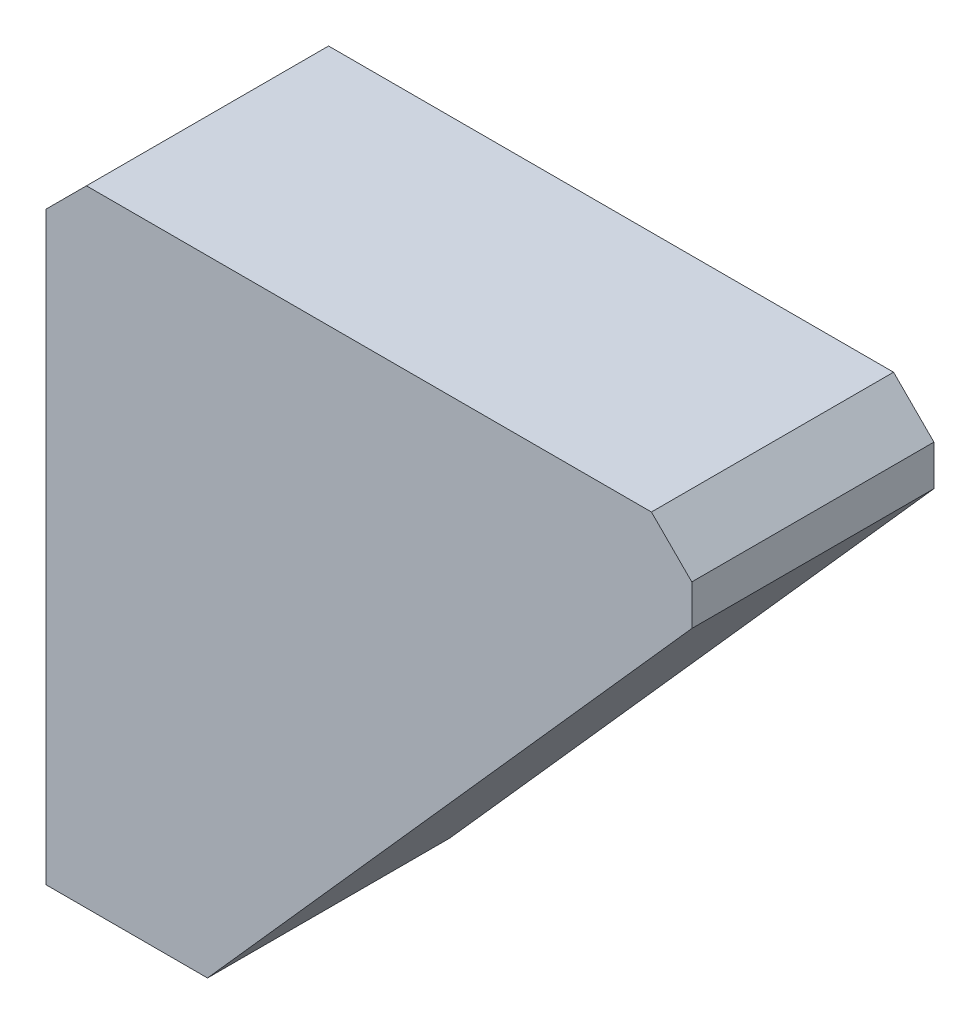
SolidWorks part; units mm, degrees
ref_plane "Front Plane" through (0, 0, 0) normal (0, 0, 1) x (1, 0, 0)
ref_plane "Top Plane" through (0, 0, 0) normal (0, 1, 0) x (1, 0, 0)
ref_plane "Right Plane" through (0, 0, 0) normal (1, 0, 0) x (0, 0, -1)
sketch "Sketch1" plane through (0, 0, 0) normal (0, 0, 1) x (1, 0, 0)
  line L0 (0, 0) -> (0, 72.5)
  line L1 (5, 77.5) -> (75, 77.5)
  line L2 (80, 72.5) -> (80, 67.5)
  line L3 (80, 67.5) -> (20, 0)
  line L4 (20, 0) -> (0, 0)
  line L5 (0, 72.5) -> (5, 77.5)
  line L6 (75, 77.5) -> (80, 72.5)
  point P1 (0, 77.5)
  point P4 (80, 77.5)
  dimension "D1" = 77.5
  dimension "D2" = 20
  dimension "D3" = 80
  dimension "D4" = 10
  dimension "D5" = 5
  dimension "D6" = 45
  dimension "D7" = 5
  dimension "D8" = 45
extrude "Boss-Extrude1" add sketch "Sketch1" along normal blind 30
